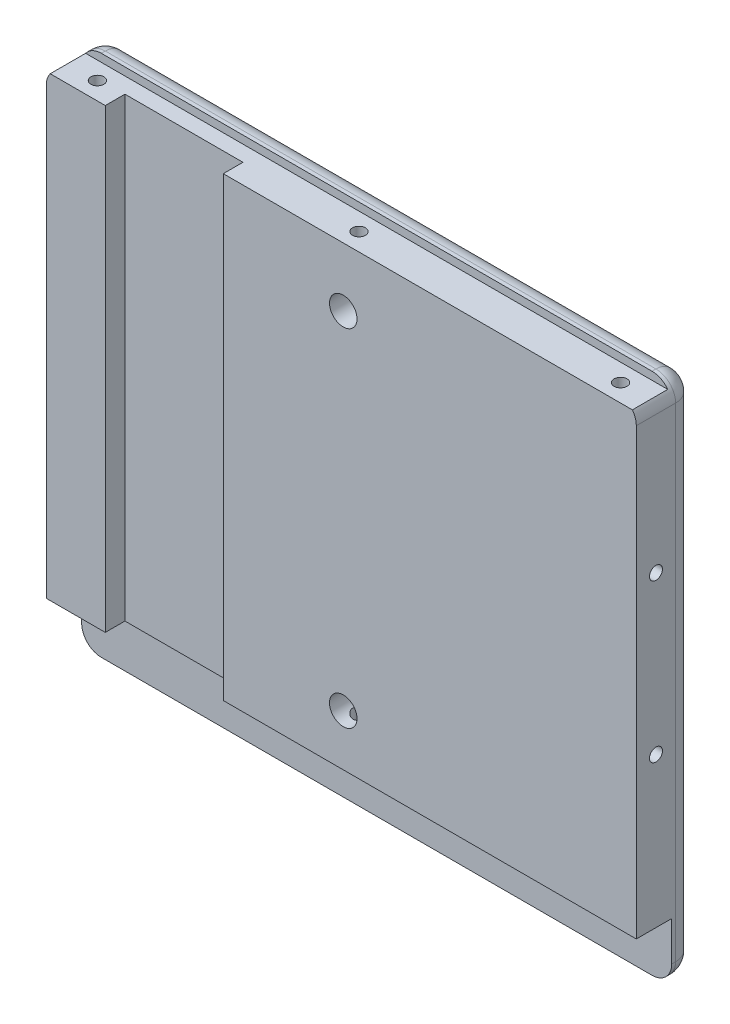
SolidWorks part; units mm, degrees
material "6061铝"
ref_plane "前视基准面" through (0, 0, 0) normal (0, 0, 1) x (1, 0, 0)
ref_plane "上视基准面" through (0, 0, 0) normal (0, 1, 0) x (1, 0, 0)
ref_plane "右视基准面" through (0, 0, 0) normal (1, 0, 0) x (0, 0, -1)
sketch "草图1" plane through (0, 0, 0) normal (0, 0, 1) x (1, 0, 0)
  line L1 (-75, 66.5) -> (75, 66.5)
  line L2 (-75, 66.5) -> (-75, -66.5)
  line L3 (-75, -66.5) -> (75, -66.5)
  line L4 (75, 66.5) -> (75, -66.5)
  line L5 (-75, 66.5) -> (75, -66.5) construction
  line L6 (-75, -66.5) -> (75, 66.5) construction
  point P0 (0, 0)
  dimension "D1" = 150
  dimension "D2" = 133
extrude "凸台-拉伸1" add sketch "草图1" along normal blind 15
sketch "草图2" plane through (-75, 0, 0) normal (-1, 0, 0) x (0, 0, 1)
  line L0 (15, 66.5) -> (15, -66.5) construction
  line L1 (29.6808, 94.726) -> (6, 94.726)
  line L2 (29.6808, 94.726) -> (29.6808, 64.5)
  line L3 (29.6808, 64.5) -> (6, 64.5)
  line L4 (6, 94.726) -> (6, 64.5)
  line L5 (29.6808, 94.726) -> (6, 64.5) construction
  line L6 (29.6808, 64.5) -> (6, 94.726) construction
  line L7 (15, 66.5) -> (0, 66.5) construction
  point P0 (17.8404, 79.613)
  dimension "D1" = 9
  dimension "D2" = 2
extrude "切除-拉伸1" cut sketch "草图2" against normal through all
fillet "圆角2" radius 5 8 edges at (-75, 66.5, 3) (-75, 0, 0) (-75, -66.5, 7.5) (0, -66.5, 0) (75, -66.5, 7.5) (75, 0, 0) (75, 66.5, 3) (0, 66.5, 0)
hole_wizard "打孔尺寸(%根据)开槽圆柱头螺钉的类型2" positions "草图6" profile "草图5" counterbore size "M6" standard "GB" end condition through all
sketch "草图6" plane through (0, 0, 0) normal (0, 0, -1) x (-1, 0, 0)
  line L0 (-70, 66.5) -> (70, 66.5) construction
  line L1 (75, 61.5) -> (75, -61.5) construction
  line L2 (70, -66.5) -> (-70, -66.5) construction
  point P0 (-0.5, 49.5)
  point P9 (-0.5, -38.5)
  dimension "D1" = 17
  dimension "D2" = 75.5
  dimension "D3" = 28
sketch "草图5" plane through (0.5, 49.5, 0) normal (1, 0, 0) x (0, 1, 0)
  line L0 (0, 0) -> (0, 15)
  line L1 (0, 15) -> (3.5, 15)
  line L3 (3.5, 15) -> (3.5, 7)
  line L4 (3.5, 7) -> (5.5, 7)
  line L5 (5.5, 7) -> (5.5, 0)
  line L7 (5.5, 0) -> (0, 0)
  line L11 (0, -6.35) -> (0, 107.95) construction
  dimension "通孔孔直径" = 7
  dimension "通孔孔深度" = 15
  dimension "柱形沉头孔直径" = 11
  dimension "柱形沉头孔深度" = 7
sketch "草图19" plane through (0, -66.5, 0) normal (0, -1, 0) x (1, 0, 0)
  line L0 (-70, 15) -> (70, 15) construction
  line L1 (-137.502, 120.666) -> (106.6005, 120.666)
  line L2 (-137.502, 120.666) -> (-137.502, 6)
  line L3 (-137.502, 6) -> (106.6005, 6)
  line L4 (106.6005, 120.666) -> (106.6005, 6)
  line L5 (-137.502, 120.666) -> (106.6005, 6) construction
  line L6 (-137.502, 6) -> (106.6005, 120.666) construction
  point P0 (-15.4508, 63.333)
  dimension "D1" = 9
extrude "切除-拉伸7" cut sketch "草图19" against normal blind 15
sketch "草图29" plane through (0, 0, 15) normal (0, 0, 1) x (1, 0, 0)
  line L1 (-60, 128.7666) -> (-30, 128.7666)
  line L2 (-60, 128.7666) -> (-60, -100.6845)
  line L3 (-60, -100.6845) -> (-30, -100.6845)
  line L4 (-30, 128.7666) -> (-30, -100.6845)
  line L5 (-60, 128.7666) -> (-30, -100.6845) construction
  line L6 (-60, -100.6845) -> (-30, 128.7666) construction
  line L7 (-75, 61.5) -> (-75, -51.5) construction
  point P0 (-45, 14.041)
  dimension "D1" = 15
  dimension "D2" = 30
extrude "切除-拉伸11" cut sketch "草图29" against normal blind 5
hole_wizard "M4 螺纹孔1" positions "草图30" profile "草图32" tap size "M4" standard "GB"
sketch "草图30" plane through (0, -51.5, 0) normal (0, -1, 0) x (-1, 0, 0)
  line L0 (0, 0) -> (0, -31.4099) construction
  line L1 (30, -15) -> (-75, -15) construction
  point P0 (66.5, -10.5)
  point P8 (-66.5, -10.5)
  point P10 (0, -10.5)
  dimension "D1" = 133
  dimension "D2" = 4.5
sketch "草图32" plane through (-66.5, -51.5, 10.5) normal (1, 0, 0) x (0, 0, -1)
  line L0 (0, 0) -> (0, 12.9914)
  line L1 (0, 12.9914) -> (1.65, 12)
  line L2 (1.65, 12) -> (1.65, 0)
  line L5 (1.65, 0) -> (0, 0)
  line L10 (0, 12.9914) -> (-1.65, 12) construction
  line L11 (0, -6.35) -> (0, 107.95) construction
  dimension "螺纹孔钻头直径" = 3.3
  dimension "螺纹孔钻头深度" = 12
  dimension "导头角度" = 118
cosmetic thread "孔螺蚊线14" parameters "D1"=8, "D2"=4
cosmetic thread "孔螺蚊线19" parameters "D1"=8, "D2"=4
cosmetic thread "孔螺蚊线21" parameters "D1"=8, "D2"=4
hole_wizard "M4 螺纹孔2" positions "草图33" profile "草图34" tap size "M4" standard "GB"
sketch "草图33" plane through (0, 64.5, 0) normal (0, 1, 0) x (1, 0, 0)
  line L0 (0, 0) -> (0, -37.5912) construction
  line L2 (-30, -15) -> (74, -15) construction
  point P0 (-66.5, -10.5)
  point P3 (66.5, -10.5)
  point P6 (0, -10.5)
  dimension "D1" = 4.5
  dimension "D2" = 133
sketch "草图34" plane through (-66.5, 64.5, 10.5) normal (1, 0, 0) x (0, 0, 1)
  line L0 (0, 0) -> (0, 12.9914)
  line L1 (0, 12.9914) -> (1.65, 12)
  line L2 (1.65, 12) -> (1.65, 0)
  line L5 (1.65, 0) -> (0, 0)
  line L10 (0, 12.9914) -> (-1.65, 12) construction
  line L11 (0, -6.35) -> (0, 107.95) construction
  dimension "螺纹孔钻头直径" = 3.3
  dimension "螺纹孔钻头深度" = 12
  dimension "导头角度" = 118
cosmetic thread "孔螺蚊线16" parameters "D1"=8, "D2"=4
cosmetic thread "孔螺蚊线17" parameters "D1"=8, "D2"=4
cosmetic thread "孔螺蚊线20" parameters "D1"=8, "D2"=4
hole_wizard "M4 螺纹孔3" positions "草图35" profile "草图37" tap size "M4" standard "GB"
sketch "草图35" plane through (-75, 0, 0) normal (-1, 0, 0) x (0, 0, 1)
  point P0 (10, 26.6108)
  point P3 (10, -13.3892)
cosmetic thread "孔螺蚊线22" parameters "D1"=8, "D2"=4
cosmetic thread "孔螺蚊线23" parameters "D1"=8, "D2"=4
sketch "草图37" plane through (-75, 26.6108, 10) normal (0, 1, 0) x (0, 0, 1)
  line L0 (0, 0) -> (0, 12.9914)
  line L1 (0, 12.9914) -> (1.65, 12)
  line L2 (1.65, 12) -> (1.65, 0)
  line L5 (1.65, 0) -> (0, 0)
  line L10 (0, 12.9914) -> (-1.65, 12) construction
  line L11 (0, -6.35) -> (0, 107.95) construction
  dimension "螺纹孔钻头直径" = 3.3
  dimension "螺纹孔钻头深度" = 12
  dimension "导头角度" = 118
mirror "镜向1" about plane through (0, 0, 0) normal (1, 0, 0) of "M4 螺纹孔3"
